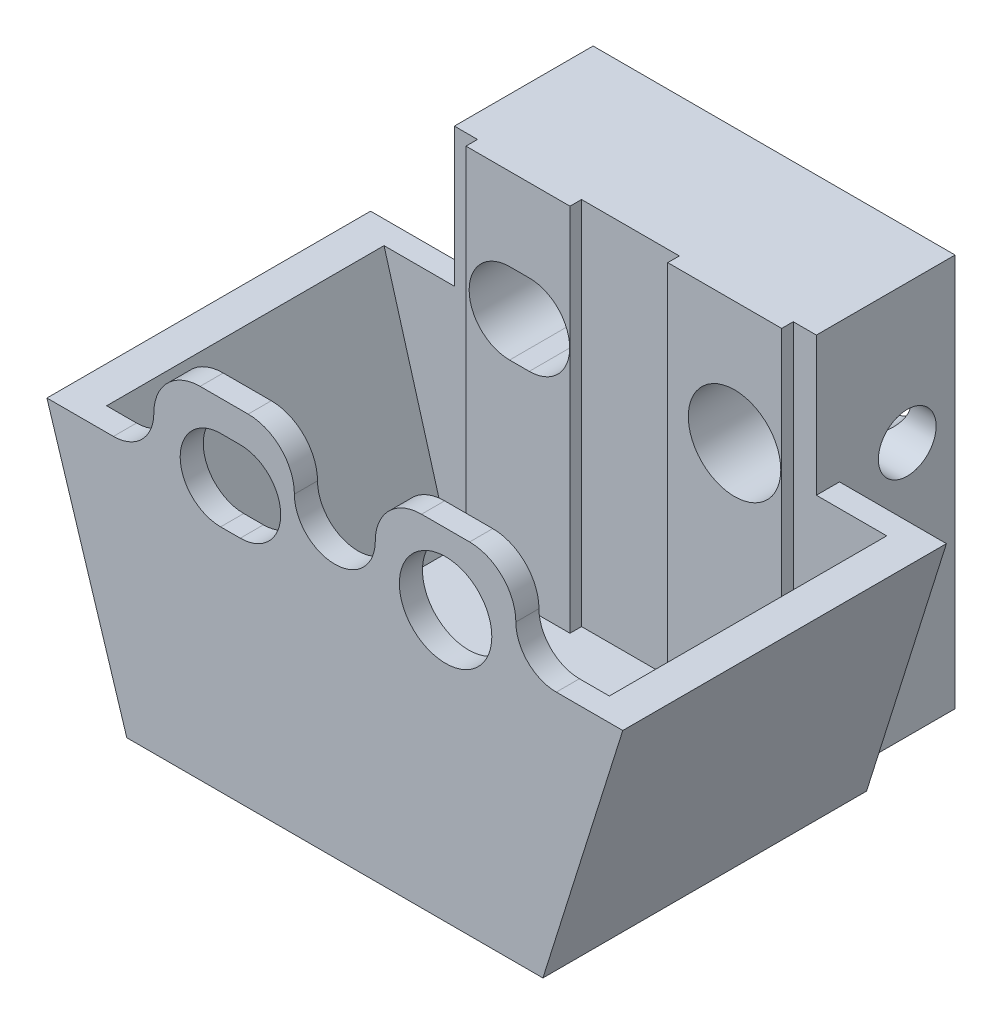
from build123d import *

# Parameters (mm, degrees)
EXTRUDE_2_DEPTH          = 140
EXTRUDE_3_DEPTH          = 140
SKETCH_8_W               = 100
SKETCH_8_H               = 240
CUT_EXTRUDE_1_DEPTH      = 275
EXTRUDE_4_DEPTH          = 100
EXTRUDE_4_DEPTH_BACK     = 20
SKETCH_12_W              = 313.16541006
SKETCH_12_H              = 120
SKETCH_13_W              = 313.16541006
SKETCH_13_H              = 220
EXTRUDE_5_DEPTH          = 100
SKETCH_14_R              = 25
CUT_EXTRUDE_2_DEPTH      = 582.186358517
SKETCH_15_W              = 90
SKETCH_15_H              = 10
SKETCH_15_W_2            = 98.58270503
EXTRUDE_6_DEPTH          = 320
CUT_EXTRUDE_3_DEPTH      = 615.919414052
CUT_EXTRUDE_3_DEPTH_BACK = 615.919414052
SKETCH_16_R              = 40


with BuildPart() as part:
    # 草图1 → 凸台-拉伸2 (new body)
    with BuildSketch(Plane.XY):
        with BuildLine():
            Line((0, 0), (180, 0))
            Line((180, 0), (180, 220))
            ThreePointArc((180, 220), (155.251262658, 230.251262658), (145, 255))
            ThreePointArc((145, 255), (133.284271247, 283.284271247), (105, 295))
            Line((105, 295), (63.41729497, 295))
            ThreePointArc((63.41729497, 295), (35.133023723, 283.284271247), (23.41729497, 255))
            ThreePointArc((23.41729497, 255), (13.166032312, 230.251262658), (-11.58270503, 220))
            Line((-11.58270503, 220), (-69.098922823, 220))
            Line((-69.098922823, 220), (0, 0))
        make_face()
    extrude_2 = extrude(amount=EXTRUDE_2_DEPTH)

    # 草图5 → 凸台-拉伸3 (add)
    with BuildSketch(Plane(origin=(0, 0, 0), x_dir=(-1, 0, 0), z_dir=(0, 0, -1))):
        Polygon((-180, 220), (69.098922823, 220), (0, 0), (-180, 0), align=None)
    extrude_3 = extrude(amount=EXTRUDE_3_DEPTH)

    # 草图8 → 切除-拉伸1 (cut)
    with BuildSketch(Plane(origin=(0, 295, 0), x_dir=(1, 0, 0), z_dir=(0, 1, 0))):
        with Locations((130, 0)):
            Rectangle(SKETCH_8_W, SKETCH_8_H)
    cut_extrude_1 = extrude(amount=-CUT_EXTRUDE_1_DEPTH, mode=Mode.SUBTRACT)

    # 草图10 → 切除-放样4 section 0
    with BuildSketch(Plane(origin=(0, 20, 0), x_dir=(1, 0, 0), z_dir=(0, 1, 0))):
        with BuildLine():
            Line((80, 120), (20, 120))
            Line((20, 120), (20, -120))
            Line((20, -120), (80, -120))
            Line((80, -120), (80, 120))
        make_face()
    # 草图11 → 切除-放样4 section 1
    with BuildSketch(Plane(origin=(0, 295, 0), x_dir=(1, 0, 0), z_dir=(0, 1, 0))):
        with BuildLine():
            Line((80, 120), (80, -120))
            Line((80, -120), (-59, -120))
            Line((-59, -120), (-59, 120))
            Line((-59, 120), (80, 120))
        make_face()
    loft_4 = loft(mode=Mode.SUBTRACT)

    # 镜向1: 凸台-拉伸2, 凸台-拉伸3, 切除-拉伸1, 切除-放样4 across plane
    add(extrude_2.mirror(Plane(origin=(180, 0, 140), x_dir=(0, 0, 1), z_dir=(-1, 0, 0))))
    add(extrude_3.mirror(Plane(origin=(180, 0, 140), x_dir=(0, 0, 1), z_dir=(-1, 0, 0))))
    add(cut_extrude_1.mirror(Plane(origin=(180, 0, 140), x_dir=(0, 0, 1), z_dir=(-1, 0, 0))), mode=Mode.SUBTRACT)
    add(loft_4.mirror(Plane(origin=(180, 0, 140), x_dir=(0, 0, 1), z_dir=(-1, 0, 0))), mode=Mode.SUBTRACT)

    # 草图12 → 凸台-拉伸4 (add, two sides: drawn at the far end of the back side and taken through both)
    with BuildSketch(Plane(origin=(0, 0, -140), x_dir=(-1, 0, 0), z_dir=(0, 0, -1)).offset(-EXTRUDE_4_DEPTH_BACK)):
        with Locations((-180, 280)):
            Rectangle(SKETCH_12_W, SKETCH_12_H)
    extrude(amount=EXTRUDE_4_DEPTH + EXTRUDE_4_DEPTH_BACK)

    # 草图13 → 凸台-拉伸5 (add)
    with BuildSketch(Plane(origin=(0, 0, -140), x_dir=(-1, 0, 0), z_dir=(0, 0, -1))):
        with Locations((-180, 110)):
            Rectangle(SKETCH_13_W, SKETCH_13_H)
    extrude(amount=EXTRUDE_5_DEPTH)

    # 草图14 → 切除-拉伸2 (cut, through all)
    with BuildSketch(Plane(origin=(336.58270503, 0, 0), x_dir=(0, 0, -1), z_dir=(1, 0, 0))):
        with Locations(Location((198.620904307, 220, 0), (0, 0, 90))):
            Circle(SKETCH_14_R)
    extrude(amount=-CUT_EXTRUDE_2_DEPTH, mode=Mode.SUBTRACT)

    # 草图15 → 凸台-拉伸6 (add)
    with BuildSketch(Plane(origin=(0, 340, 0), x_dir=(1, 0, 0), z_dir=(0, 1, 0))):
        with Locations((88.41729497, 115)):
            Rectangle(SKETCH_15_W, SKETCH_15_H)
        with Locations((267.291352515, 115)):
            Rectangle(SKETCH_15_W_2, SKETCH_15_H)
    extrude(amount=-EXTRUDE_6_DEPTH)

    # 草图16 → 切除-拉伸3 (cut, two sides: drawn at the far end of the back side and taken through both)
    with BuildSketch(Plane(origin=(0, 0, -140), x_dir=(-1, 0, 0), z_dir=(0, 0, -1)).offset(-CUT_EXTRUDE_3_DEPTH_BACK)):
        with Locations(Location((-275.791352515, 233.606267036, 0), (0, 0, 90))):
            Circle(SKETCH_16_R)
        with BuildLine():
            Line((-98.176420136, 268.606267036), (-81.17642014, 268.606267036))
            ThreePointArc((-81.17642014, 268.606267036), (-46.17642014, 233.606267036), (-81.17642014, 198.606267036))
            Line((-81.17642014, 198.606267036), (-98.176420136, 198.606267036))
            ThreePointArc((-98.176420136, 198.606267036), (-133.176420136, 233.606267036), (-98.176420136, 268.606267036))
        make_face()
    extrude(amount=CUT_EXTRUDE_3_DEPTH + CUT_EXTRUDE_3_DEPTH_BACK, mode=Mode.SUBTRACT)


solid = part.part
